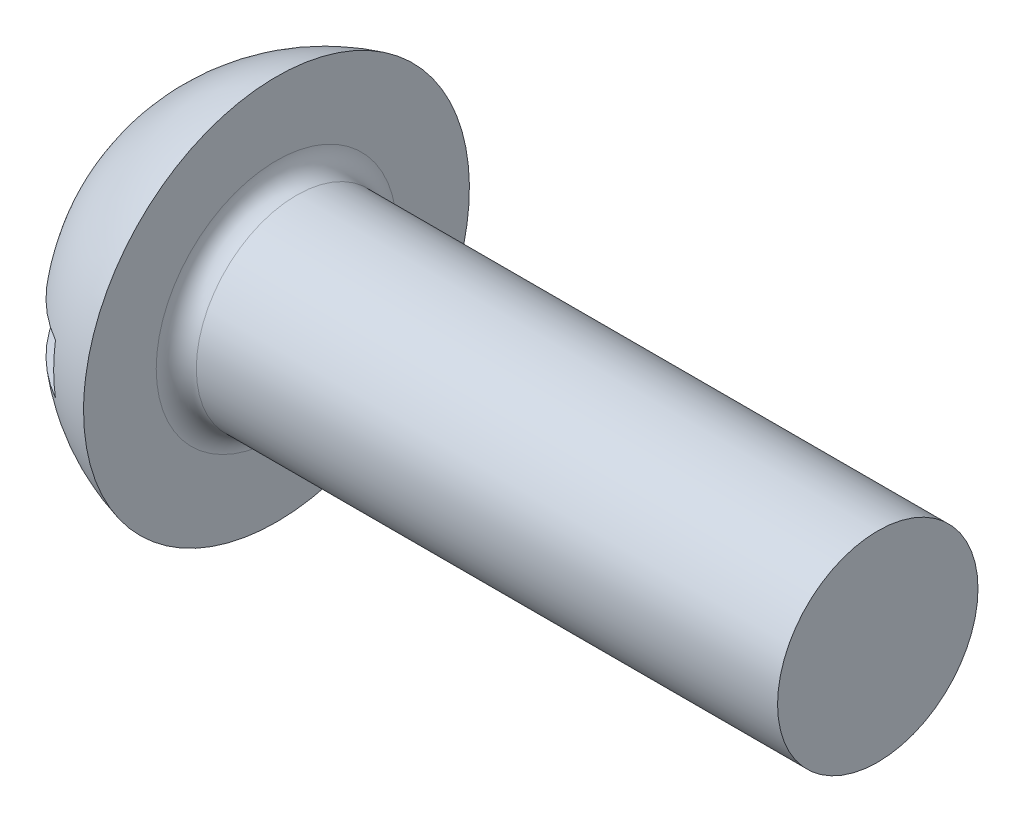
from build123d import *

# Parameters (mm, degrees)
SKETCH_2_W          = 7.7
SKETCH_2_H          = 1
CUT_EXTRUDE_1_DEPTH = 2
FILLET_1_R          = 0.4


with BuildPart() as part:
    # 草图1 → 旋转1 (revolve)
    with BuildSketch(Plane.XY):
        with BuildLine():
            Line((3, 3.85), (3, 2))
            Line((3, 2), (7, 2))
            Line((7, 2), (15, 2))
            Line((15, 2), (15, 0))
            Line((15, 0), (0, 0))
            ThreePointArc((0, 0), (0.838550848, 2.440414924), (3, 3.85))
        make_face()
    revolve(axis=Axis((0, 0, 0), (1, 0, 0)))

    # 草图2 → 切除-拉伸1 (cut)
    with BuildSketch(Plane(origin=(0, 0, 0), x_dir=(0, 0, -1), z_dir=(1, 0, 0))):
        Rectangle(SKETCH_2_W, SKETCH_2_H)
    extrude(amount=CUT_EXTRUDE_1_DEPTH, mode=Mode.SUBTRACT)

    # 圆角1
    fillet_1_edges = [part.edges().sort_by_distance(p)[0] for p in [
        (3, -2, 0),
    ]]
    fillet(fillet_1_edges, radius=FILLET_1_R)


solid = part.part
